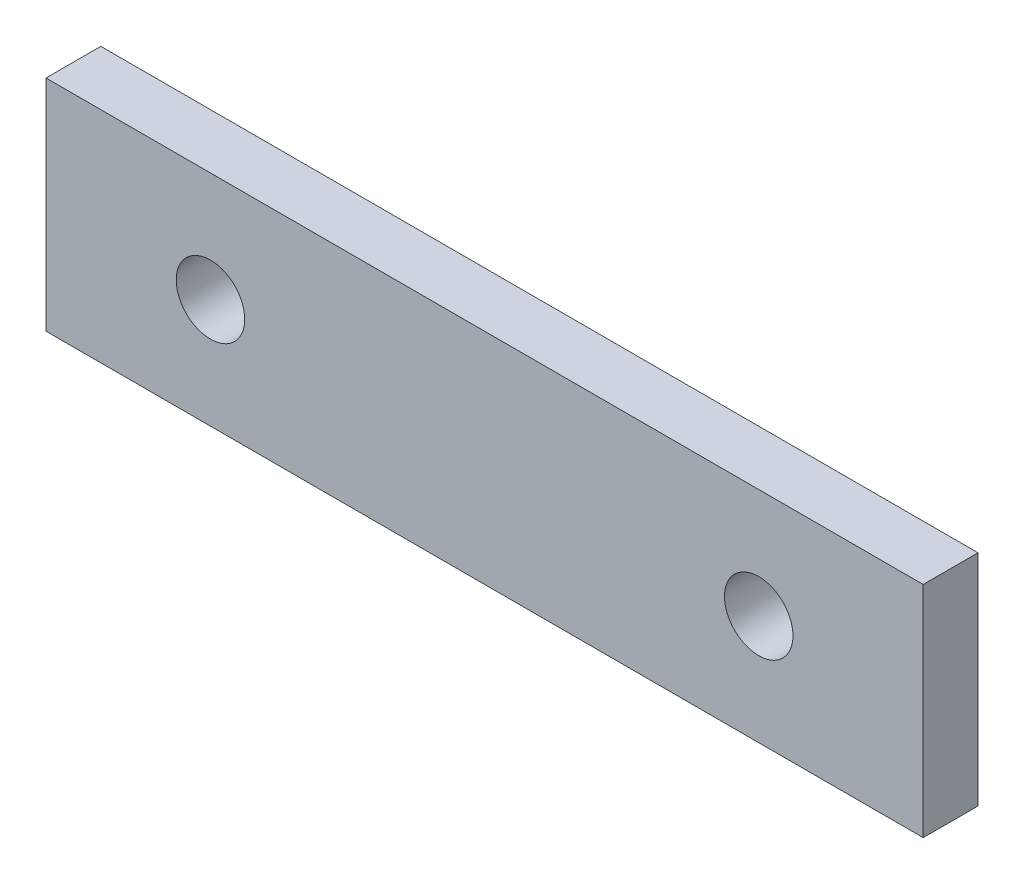
from build123d import *

# Parameters (mm, degrees)
SKETCH1_W                    = 160
SKETCH1_H                    = 40
BOSS_EXTRUDE1_DEPTH          = 5
F_12_5_12_5_DIAMETER_HOLE1_D = 12.5


with BuildPart() as part:
    # Sketch1 → Boss-Extrude1 (new, symmetric)
    with BuildSketch(Plane.XY):
        Rectangle(SKETCH1_W, SKETCH1_H)
    extrude(amount=BOSS_EXTRUDE1_DEPTH, both=True)

    # Ø12.5 (12.5) Diameter Hole1 (through all)
    with Locations(Plane.XY.offset(5)):
        with Locations((-50, 0), (50, 0)):
            Hole(F_12_5_12_5_DIAMETER_HOLE1_D / 2)


solid = part.part
